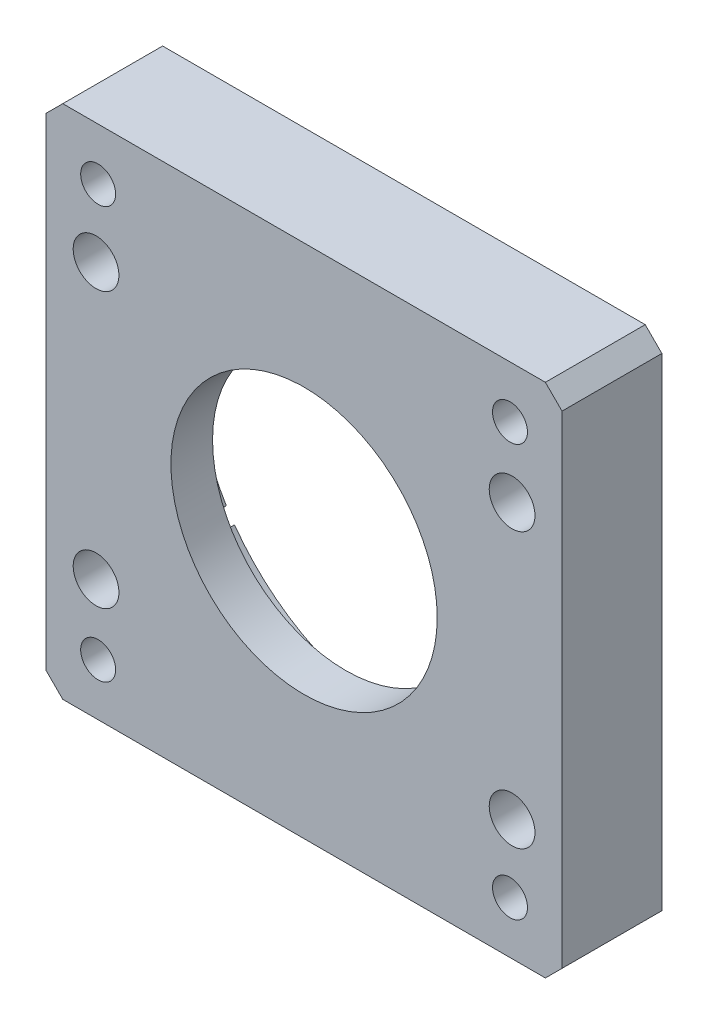
SolidWorks part; units mm, degrees
material "6061Al"
ref_plane "前视基准面" through (0, 0, 0) normal (0, 0, 1) x (1, 0, 0)
ref_plane "上视基准面" through (0, 0, 0) normal (0, 1, 0) x (1, 0, 0)
ref_plane "右视基准面" through (0, 0, 0) normal (1, 0, 0) x (0, 0, -1)
sketch "草图1" plane through (0, 0, 0) normal (0, 0, 1) x (1, 0, 0)
  line L1 (-31, -31) -> (31, -31)
  line L2 (-31, -31) -> (-31, 31)
  line L3 (-31, 31) -> (31, 31)
  line L4 (31, -31) -> (31, 31)
  line L5 (-31, -31) -> (31, 31) construction
  line L6 (-31, 31) -> (31, -31) construction
  point P0 (0, 0)
  dimension "D1" = 62
  dimension "D2" = 62
extrude "凸台-拉伸1" add sketch "草图1" along normal mid plane 12
sketch "草图2" plane through (0, 0, 6) normal (0, 0, 1) x (1, 0, 0)
  circle A0 centre (0, 0) radius 16
  dimension "D1" = 32
extrude "切除-拉伸1" cut sketch "草图2" against normal through all
hole_wizard "M5 螺纹孔1" positions "草图6" profile "草图5" tap size "M5" standard "ISO" end condition through all
sketch "草图6" plane through (0, 0, -6) normal (0, 0, 1) x (1, 0, 0)
  line L1 (-24.7487, -24.7487) -> (24.7487, -24.7487)
  line L2 (-24.7487, -24.7487) -> (-24.7487, 24.7487)
  line L3 (-24.7487, 24.7487) -> (24.7487, 24.7487)
  line L4 (24.7487, -24.7487) -> (24.7487, 24.7487)
  line L5 (-24.7487, -24.7487) -> (24.7487, 24.7487) construction
  line L6 (-24.7487, 24.7487) -> (24.7487, -24.7487) construction
  point P0 (-24.7487, 24.7487)
  point P4 (24.7487, 24.7487)
  point P7 (-24.7487, -24.7487)
  point P9 (24.7487, -24.7487)
sketch "草图5" plane through (-24.7487, 24.7487, -6) normal (1, 0, 0) x (0, 1, 0)
  line L0 (0, 0) -> (0, 12)
  line L1 (0, 12) -> (2.1, 12)
  line L2 (2.1, 12) -> (2.1, 0)
  line L5 (2.1, 0) -> (0, 0)
  line L11 (0, -6.35) -> (0, 107.95) construction
  dimension "通孔螺纹孔钻头直径" = 4.2
  dimension "通孔螺纹孔钻头深度" = 12
sketch "草图11" plane through (0, 0, -6) normal (0, 0, -1) x (-1, 0, 0)
  circle A0 centre (0, 0) radius 25
  dimension "D1" = 50
extrude "切除-拉伸2" cut sketch "草图11" against normal blind 7
hole_wizard "M5 六角凹头螺钉的柱形沉头孔1" positions "草图10" profile "草图9" counterbore size "M5" standard "ISO" end condition through all
sketch "草图10" plane through (0, 0, -6) normal (0, 0, -1) x (-1, 0, 0)
  line L0 (0, 0) -> (0, 31) construction
  line L1 (-31, 31) -> (31, 31) construction
  line L3 (0, 0) -> (31, 0) construction
  line L4 (31, 31) -> (31, -31) construction
  point P151 (-25, 16.5)
  point P168 (25, 16.5)
  point P169 (25, -16.5)
  point P170 (-25, -16.5)
  dimension "D1" = 50
  dimension "D2" = 33
sketch "草图9" plane through (25, 16.5, -6) normal (1, 0, 0) x (0, 1, 0)
  line L0 (0, 0) -> (0, 12)
  line L1 (0, 12) -> (2.75, 12)
  line L3 (2.75, 12) -> (2.75, 5.4)
  line L4 (2.75, 5.4) -> (5.05, 5.4)
  line L5 (5.05, 5.4) -> (5.05, 0)
  line L7 (5.05, 0) -> (0, 0)
  line L11 (0, -6.35) -> (0, 107.95) construction
  dimension "通孔孔直径" = 5.5
  dimension "通孔孔深度" = 12
  dimension "柱形沉头孔直径" = 10.1
  dimension "柱形沉头孔深度" = 5.4
chamfer "倒角1" distance 2 angle 45 4 edges at (-31, -31, 0) (31, -31, 0) (31, 31, 0) (-31, 31, 0)
sketch "草图13" plane through (0, 0, 1) normal (0, 0, -1) x (-1, 0, 0)
  circle A0 centre (0, 0) radius 18 construction
  circle A1 centre (0, 0) radius 19.2
  circle A2 centre (0, 0) radius 16.8
  dimension "D1" = 36
  dimension "D2" = 1.2
  dimension "D3" = 1.2
extrude "切除-拉伸3" cut sketch "草图13" against normal blind 1.5
